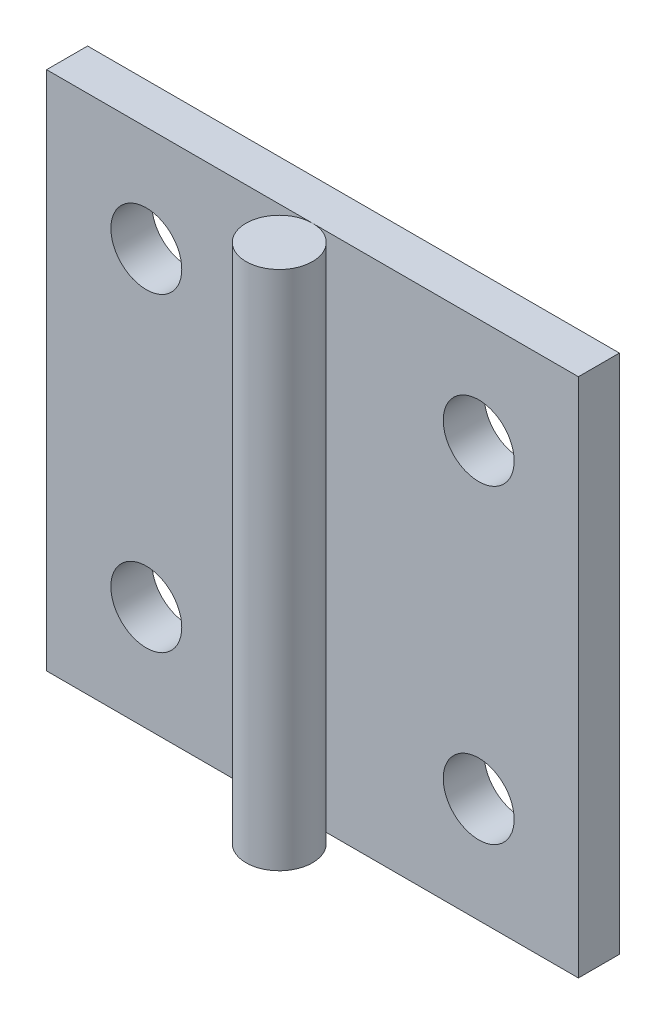
SolidWorks part; units mm, degrees
ref_plane "前视基准面" through (0, 0, 0) normal (0, 0, 1) x (1, 0, 0)
ref_plane "上视基准面" through (0, 0, 0) normal (0, 1, 0) x (1, 0, 0)
ref_plane "右视基准面" through (0, 0, 0) normal (1, 0, 0) x (0, 0, -1)
sketch "草图1" plane through (0, 0, 0) normal (0, 0, 1) x (1, 0, 0)
  line L0 (-15, 14) -> (-15, -14) construction
  line L1 (-24, 23.5) -> (24, 23.5)
  line L2 (-24, 23.5) -> (-24, -23.5)
  line L3 (-24, -23.5) -> (24, -23.5)
  line L4 (24, 23.5) -> (24, -23.5)
  line L5 (-24, 23.5) -> (24, -23.5) construction
  line L6 (-24, -23.5) -> (24, 23.5) construction
  line L7 (-15, 14) -> (15, 14) construction
  circle A0 centre (-15, 14) radius 3.2
  circle A1 centre (-15, -14) radius 3.2
  circle A2 centre (15, 14) radius 3.2
  circle A3 centre (15, -14) radius 3.2
  point P0 (0, 0)
  point P12 (-15, 0)
  point P13 (0, 14)
  dimension "D3" = 6.4
  dimension "D4" = 6.4
  dimension "D6" = 6.4
  dimension "D8" = 6.4
  dimension "D1" = 48
  dimension "D2" = 47
  dimension "D5" = 28
  dimension "D7" = 30
extrude "凸台-拉伸1" add sketch "草图1" along normal blind 3.7
sketch "草图2" plane through (0, -23.5, 0) normal (0, -1, 0) x (1, 0, 0)
  line L0 (-24, 3.7) -> (24, 3.7) construction
  circle A0 centre (0, 6.7) radius 3
  dimension "D1" = 6
  dimension "D2" = 3
extrude "凸台-拉伸2" add sketch "草图2" against normal up to surface (47 mm away) separate body up to face at (0, 23.5, 1.85)
